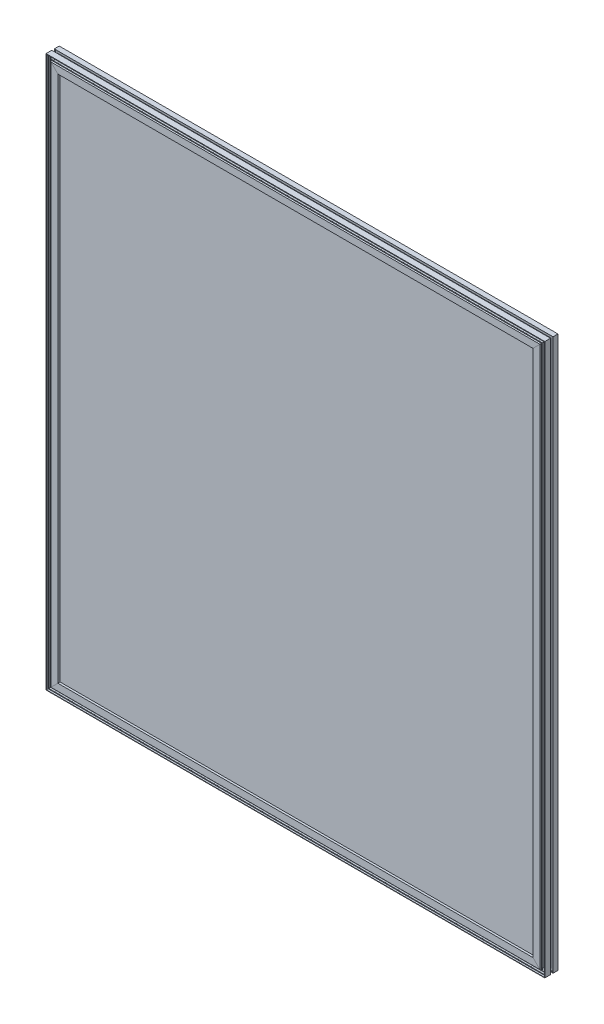
from build123d import *

# Parameters (mm, degrees)
MEMBER_250403_1_DEPTH      = 41.360872141
MEMBER_250403_1_DEPTH_BACK = 1301.360872141
MEMBER_250403_1_2_DEPTH    = 1222.721744282
MEMBER_250403_1_3_DEPTH    = 1342.721744282
MEMBER_250403_1_4_DEPTH    = 1222.721744282
SKETCH_12_W                = 1100
SKETCH_12_H                = 1220
EXTRUDE_1_DEPTH            = 17


with BuildPart() as part:
    # 草图11 → Member 250403_1 (new, two sides: drawn at the far end of the back side and taken through both)
    with BuildSketch(Plane(origin=(-570, 630, 0), x_dir=(1, 0, 0), z_dir=(0, 1, 0)).offset(-MEMBER_250403_1_DEPTH_BACK)):
        with BuildLine():
            Line((11.006838108, 0), (27, 0))
            Line((27, 0), (27, 5))
            Line((27, 5), (25.5, 5))
            Line((25.5, 5), (25.5, 2.2))
            ThreePointArc((25.5, 2.2), (25.207106781, 1.492893219), (24.5, 1.2))
            Line((24.5, 1.2), (18, 1.2))
            ThreePointArc((18, 1.2), (17.292893219, 1.492893219), (17, 2.2))
            Line((17, 2.2), (17, 30))
            Line((17, 30), (12.5, 30))
            Line((12.5, 30), (12.5, 28.8))
            Line((12.5, 28.8), (15.8, 28.8))
            Line((15.8, 28.8), (15.8, 22))
            Line((15.8, 22), (1.2, 22))
            Line((1.2, 22), (1.2, 28.8))
            Line((1.2, 28.8), (4.5, 28.8))
            Line((4.5, 28.8), (4.5, 30))
            Line((4.5, 30), (0, 30))
            Line((0, 30), (0, 18.8))
            Line((0, 18.8), (1.2, 18.8))
            Line((1.2, 18.8), (1.2, 20.8))
            Line((1.2, 20.8), (6.7, 20.8))
            Line((6.7, 20.8), (6.7, 18.8))
            Line((6.7, 18.8), (7.7, 18.8))
            Line((7.7, 18.8), (7.7, 13))
            Line((7.7, 13), (6.7, 13))
            Line((6.7, 13), (6.7, 11))
            Line((6.7, 11), (1.2, 11))
            Line((1.2, 11), (1.2, 13))
            Line((1.2, 13), (0, 13))
            Line((0, 13), (0, 0))
            Line((0, 0), (1.006838108, 0))
            Line((1.006838108, 0), (2.380431303, 2.400675266))
            ThreePointArc((2.380431303, 2.400675266), (2.379848147, 2.600337065), (2.206838108, 2.7))
            Line((2.206838108, 2.7), (1.706838108, 2.7))
            Line((1.706838108, 2.7), (1.706838108, 2.9))
            Line((1.706838108, 2.9), (2.675186721, 3.252126768))
            ThreePointArc((2.675186721, 3.252126768), (2.770651604, 3.325346014), (2.806838108, 3.440085453))
            Line((2.806838108, 3.440085453), (2.806838108, 3.9))
            ThreePointArc((2.806838108, 3.9), (2.748259465, 4.041421356), (2.606838108, 4.1))
            Line((2.606838108, 4.1), (1.006838108, 4.1))
            Line((1.006838108, 4.1), (1.006838108, 9.5))
            ThreePointArc((1.006838108, 9.5), (1.153284718, 9.853553391), (1.506838108, 10))
            Line((1.506838108, 10), (10.506838108, 10))
            ThreePointArc((10.506838108, 10), (10.860391499, 9.853553391), (11.006838108, 9.5))
            Line((11.006838108, 9.5), (11.006838108, 4.1))
            Line((11.006838108, 4.1), (9.406838108, 4.1))
            ThreePointArc((9.406838108, 4.1), (9.265416752, 4.041421356), (9.206838108, 3.9))
            Line((9.206838108, 3.9), (9.206838108, 3.440085453))
            ThreePointArc((9.206838108, 3.440085453), (9.243024613, 3.325346014), (9.338489496, 3.252126768))
            Line((9.338489496, 3.252126768), (10.306838108, 2.9))
            Line((10.306838108, 2.9), (10.306838108, 2.7))
            Line((10.306838108, 2.7), (9.806838108, 2.7))
            ThreePointArc((9.806838108, 2.7), (9.63382807, 2.600337065), (9.633244913, 2.400675266))
            Line((9.633244913, 2.400675266), (11.006838108, 0))
        make_face()
        with BuildLine():
            Line((7.9, 11), (7.9, 11.8))
            ThreePointArc((7.9, 11.8), (8.607106781, 12.092893219), (8.9, 12.8))
            Line((8.9, 12.8), (8.9, 19))
            ThreePointArc((8.9, 19), (8.607106781, 19.707106781), (7.9, 20))
            Line((7.9, 20), (7.9, 20.8))
            Line((7.9, 20.8), (16, 20.8))
            Line((16, 20.8), (16, 1.2))
            Line((16, 1.2), (12.006838108, 1.2))
            Line((12.006838108, 1.2), (12.006838108, 11))
            Line((12.006838108, 11), (7.9, 11))
        make_face(mode=Mode.SUBTRACT)
    extrude(amount=MEMBER_250403_1_DEPTH + MEMBER_250403_1_DEPTH_BACK)

    # Member 250403_1 mitre 1
    split(bisect_by=Plane(origin=(-570, 630, 0), x_dir=(0.707106781, -0.707106781, 0), z_dir=(-0.707106781, -0.707106781, 0)), keep=Keep.TOP)

    # Member 250403_1 mitre 2
    split(bisect_by=Plane(origin=(-570, -630, 0), x_dir=(-0.707106781, -0.707106781, 0), z_dir=(-0.707106781, 0.707106781, 0)), keep=Keep.TOP)


with BuildPart() as body_2:
    # 草图11 on segment 2 (carried to segment 2) → Member 250403_1 2 (new body)
    with BuildSketch(Plane(origin=(611.360872141, -630, 0), x_dir=(0, 1, 0), z_dir=(-1, 0, 0))):
        with BuildLine():
            Line((11.006838108, 0), (27, 0))
            Line((27, 0), (27, 5))
            Line((27, 5), (25.5, 5))
            Line((25.5, 5), (25.5, 2.2))
            ThreePointArc((25.5, 2.2), (25.207106781, 1.492893219), (24.5, 1.2))
            Line((24.5, 1.2), (18, 1.2))
            ThreePointArc((18, 1.2), (17.292893219, 1.492893219), (17, 2.2))
            Line((17, 2.2), (17, 30))
            Line((17, 30), (12.5, 30))
            Line((12.5, 30), (12.5, 28.8))
            Line((12.5, 28.8), (15.8, 28.8))
            Line((15.8, 28.8), (15.8, 22))
            Line((15.8, 22), (1.2, 22))
            Line((1.2, 22), (1.2, 28.8))
            Line((1.2, 28.8), (4.5, 28.8))
            Line((4.5, 28.8), (4.5, 30))
            Line((4.5, 30), (0, 30))
            Line((0, 30), (0, 18.8))
            Line((0, 18.8), (1.2, 18.8))
            Line((1.2, 18.8), (1.2, 20.8))
            Line((1.2, 20.8), (6.7, 20.8))
            Line((6.7, 20.8), (6.7, 18.8))
            Line((6.7, 18.8), (7.7, 18.8))
            Line((7.7, 18.8), (7.7, 13))
            Line((7.7, 13), (6.7, 13))
            Line((6.7, 13), (6.7, 11))
            Line((6.7, 11), (1.2, 11))
            Line((1.2, 11), (1.2, 13))
            Line((1.2, 13), (0, 13))
            Line((0, 13), (0, 0))
            Line((0, 0), (1.006838108, 0))
            Line((1.006838108, 0), (2.380431303, 2.400675266))
            ThreePointArc((2.380431303, 2.400675266), (2.379848147, 2.600337065), (2.206838108, 2.7))
            Line((2.206838108, 2.7), (1.706838108, 2.7))
            Line((1.706838108, 2.7), (1.706838108, 2.9))
            Line((1.706838108, 2.9), (2.675186721, 3.252126768))
            ThreePointArc((2.675186721, 3.252126768), (2.770651604, 3.325346014), (2.806838108, 3.440085453))
            Line((2.806838108, 3.440085453), (2.806838108, 3.9))
            ThreePointArc((2.806838108, 3.9), (2.748259465, 4.041421356), (2.606838108, 4.1))
            Line((2.606838108, 4.1), (1.006838108, 4.1))
            Line((1.006838108, 4.1), (1.006838108, 9.5))
            ThreePointArc((1.006838108, 9.5), (1.153284718, 9.853553391), (1.506838108, 10))
            Line((1.506838108, 10), (10.506838108, 10))
            ThreePointArc((10.506838108, 10), (10.860391499, 9.853553391), (11.006838108, 9.5))
            Line((11.006838108, 9.5), (11.006838108, 4.1))
            Line((11.006838108, 4.1), (9.406838108, 4.1))
            ThreePointArc((9.406838108, 4.1), (9.265416752, 4.041421356), (9.206838108, 3.9))
            Line((9.206838108, 3.9), (9.206838108, 3.440085453))
            ThreePointArc((9.206838108, 3.440085453), (9.243024613, 3.325346014), (9.338489496, 3.252126768))
            Line((9.338489496, 3.252126768), (10.306838108, 2.9))
            Line((10.306838108, 2.9), (10.306838108, 2.7))
            Line((10.306838108, 2.7), (9.806838108, 2.7))
            ThreePointArc((9.806838108, 2.7), (9.63382807, 2.600337065), (9.633244913, 2.400675266))
            Line((9.633244913, 2.400675266), (11.006838108, 0))
        make_face()
        with BuildLine():
            Line((7.9, 11), (7.9, 11.8))
            ThreePointArc((7.9, 11.8), (8.607106781, 12.092893219), (8.9, 12.8))
            Line((8.9, 12.8), (8.9, 19))
            ThreePointArc((8.9, 19), (8.607106781, 19.707106781), (7.9, 20))
            Line((7.9, 20), (7.9, 20.8))
            Line((7.9, 20.8), (16, 20.8))
            Line((16, 20.8), (16, 1.2))
            Line((16, 1.2), (12.006838108, 1.2))
            Line((12.006838108, 1.2), (12.006838108, 11))
            Line((12.006838108, 11), (7.9, 11))
        make_face(mode=Mode.SUBTRACT)
    extrude(amount=MEMBER_250403_1_2_DEPTH)

    # Member 250403_1 2 mitre 1
    split(bisect_by=Plane(origin=(-570, -630, 0), x_dir=(0.707106781, 0.707106781, 0), z_dir=(0.707106781, -0.707106781, 0)), keep=Keep.TOP)

    # Member 250403_1 2 mitre 2
    split(bisect_by=Plane(origin=(570, -630, 0), x_dir=(0.707106781, -0.707106781, 0), z_dir=(-0.707106781, -0.707106781, 0)), keep=Keep.TOP)


with BuildPart() as body_3:
    # 草图11 on segment 3 (carried to segment 3) → Member 250403_1 3 (new body)
    with BuildSketch(Plane(origin=(570, 671.360872141, 0), x_dir=(-1, 0, 0), z_dir=(0, -1, 0))):
        with BuildLine():
            Line((11.006838108, 0), (27, 0))
            Line((27, 0), (27, 5))
            Line((27, 5), (25.5, 5))
            Line((25.5, 5), (25.5, 2.2))
            ThreePointArc((25.5, 2.2), (25.207106781, 1.492893219), (24.5, 1.2))
            Line((24.5, 1.2), (18, 1.2))
            ThreePointArc((18, 1.2), (17.292893219, 1.492893219), (17, 2.2))
            Line((17, 2.2), (17, 30))
            Line((17, 30), (12.5, 30))
            Line((12.5, 30), (12.5, 28.8))
            Line((12.5, 28.8), (15.8, 28.8))
            Line((15.8, 28.8), (15.8, 22))
            Line((15.8, 22), (1.2, 22))
            Line((1.2, 22), (1.2, 28.8))
            Line((1.2, 28.8), (4.5, 28.8))
            Line((4.5, 28.8), (4.5, 30))
            Line((4.5, 30), (0, 30))
            Line((0, 30), (0, 18.8))
            Line((0, 18.8), (1.2, 18.8))
            Line((1.2, 18.8), (1.2, 20.8))
            Line((1.2, 20.8), (6.7, 20.8))
            Line((6.7, 20.8), (6.7, 18.8))
            Line((6.7, 18.8), (7.7, 18.8))
            Line((7.7, 18.8), (7.7, 13))
            Line((7.7, 13), (6.7, 13))
            Line((6.7, 13), (6.7, 11))
            Line((6.7, 11), (1.2, 11))
            Line((1.2, 11), (1.2, 13))
            Line((1.2, 13), (0, 13))
            Line((0, 13), (0, 0))
            Line((0, 0), (1.006838108, 0))
            Line((1.006838108, 0), (2.380431303, 2.400675266))
            ThreePointArc((2.380431303, 2.400675266), (2.379848147, 2.600337065), (2.206838108, 2.7))
            Line((2.206838108, 2.7), (1.706838108, 2.7))
            Line((1.706838108, 2.7), (1.706838108, 2.9))
            Line((1.706838108, 2.9), (2.675186721, 3.252126768))
            ThreePointArc((2.675186721, 3.252126768), (2.770651604, 3.325346014), (2.806838108, 3.440085453))
            Line((2.806838108, 3.440085453), (2.806838108, 3.9))
            ThreePointArc((2.806838108, 3.9), (2.748259465, 4.041421356), (2.606838108, 4.1))
            Line((2.606838108, 4.1), (1.006838108, 4.1))
            Line((1.006838108, 4.1), (1.006838108, 9.5))
            ThreePointArc((1.006838108, 9.5), (1.153284718, 9.853553391), (1.506838108, 10))
            Line((1.506838108, 10), (10.506838108, 10))
            ThreePointArc((10.506838108, 10), (10.860391499, 9.853553391), (11.006838108, 9.5))
            Line((11.006838108, 9.5), (11.006838108, 4.1))
            Line((11.006838108, 4.1), (9.406838108, 4.1))
            ThreePointArc((9.406838108, 4.1), (9.265416752, 4.041421356), (9.206838108, 3.9))
            Line((9.206838108, 3.9), (9.206838108, 3.440085453))
            ThreePointArc((9.206838108, 3.440085453), (9.243024613, 3.325346014), (9.338489496, 3.252126768))
            Line((9.338489496, 3.252126768), (10.306838108, 2.9))
            Line((10.306838108, 2.9), (10.306838108, 2.7))
            Line((10.306838108, 2.7), (9.806838108, 2.7))
            ThreePointArc((9.806838108, 2.7), (9.63382807, 2.600337065), (9.633244913, 2.400675266))
            Line((9.633244913, 2.400675266), (11.006838108, 0))
        make_face()
        with BuildLine():
            Line((7.9, 11), (7.9, 11.8))
            ThreePointArc((7.9, 11.8), (8.607106781, 12.092893219), (8.9, 12.8))
            Line((8.9, 12.8), (8.9, 19))
            ThreePointArc((8.9, 19), (8.607106781, 19.707106781), (7.9, 20))
            Line((7.9, 20), (7.9, 20.8))
            Line((7.9, 20.8), (16, 20.8))
            Line((16, 20.8), (16, 1.2))
            Line((16, 1.2), (12.006838108, 1.2))
            Line((12.006838108, 1.2), (12.006838108, 11))
            Line((12.006838108, 11), (7.9, 11))
        make_face(mode=Mode.SUBTRACT)
    extrude(amount=MEMBER_250403_1_3_DEPTH)

    # Member 250403_1 3 mitre 1
    split(bisect_by=Plane(origin=(570, 630, 0), x_dir=(0.707106781, 0.707106781, 0), z_dir=(0.707106781, -0.707106781, 0)), keep=Keep.TOP)

    # Member 250403_1 3 mitre 2
    split(bisect_by=Plane(origin=(570, -630, 0), x_dir=(-0.707106781, 0.707106781, 0), z_dir=(0.707106781, 0.707106781, 0)), keep=Keep.TOP)


with BuildPart() as body_4:
    # 草图11 on segment 4 (carried to segment 4) → Member 250403_1 4 (new body)
    with BuildSketch(Plane(origin=(-611.360872141, 630, 0), x_dir=(0, -1, 0), z_dir=(1, 0, 0))):
        with BuildLine():
            Line((11.006838108, 0), (27, 0))
            Line((27, 0), (27, 5))
            Line((27, 5), (25.5, 5))
            Line((25.5, 5), (25.5, 2.2))
            ThreePointArc((25.5, 2.2), (25.207106781, 1.492893219), (24.5, 1.2))
            Line((24.5, 1.2), (18, 1.2))
            ThreePointArc((18, 1.2), (17.292893219, 1.492893219), (17, 2.2))
            Line((17, 2.2), (17, 30))
            Line((17, 30), (12.5, 30))
            Line((12.5, 30), (12.5, 28.8))
            Line((12.5, 28.8), (15.8, 28.8))
            Line((15.8, 28.8), (15.8, 22))
            Line((15.8, 22), (1.2, 22))
            Line((1.2, 22), (1.2, 28.8))
            Line((1.2, 28.8), (4.5, 28.8))
            Line((4.5, 28.8), (4.5, 30))
            Line((4.5, 30), (0, 30))
            Line((0, 30), (0, 18.8))
            Line((0, 18.8), (1.2, 18.8))
            Line((1.2, 18.8), (1.2, 20.8))
            Line((1.2, 20.8), (6.7, 20.8))
            Line((6.7, 20.8), (6.7, 18.8))
            Line((6.7, 18.8), (7.7, 18.8))
            Line((7.7, 18.8), (7.7, 13))
            Line((7.7, 13), (6.7, 13))
            Line((6.7, 13), (6.7, 11))
            Line((6.7, 11), (1.2, 11))
            Line((1.2, 11), (1.2, 13))
            Line((1.2, 13), (0, 13))
            Line((0, 13), (0, 0))
            Line((0, 0), (1.006838108, 0))
            Line((1.006838108, 0), (2.380431303, 2.400675266))
            ThreePointArc((2.380431303, 2.400675266), (2.379848147, 2.600337065), (2.206838108, 2.7))
            Line((2.206838108, 2.7), (1.706838108, 2.7))
            Line((1.706838108, 2.7), (1.706838108, 2.9))
            Line((1.706838108, 2.9), (2.675186721, 3.252126768))
            ThreePointArc((2.675186721, 3.252126768), (2.770651604, 3.325346014), (2.806838108, 3.440085453))
            Line((2.806838108, 3.440085453), (2.806838108, 3.9))
            ThreePointArc((2.806838108, 3.9), (2.748259465, 4.041421356), (2.606838108, 4.1))
            Line((2.606838108, 4.1), (1.006838108, 4.1))
            Line((1.006838108, 4.1), (1.006838108, 9.5))
            ThreePointArc((1.006838108, 9.5), (1.153284718, 9.853553391), (1.506838108, 10))
            Line((1.506838108, 10), (10.506838108, 10))
            ThreePointArc((10.506838108, 10), (10.860391499, 9.853553391), (11.006838108, 9.5))
            Line((11.006838108, 9.5), (11.006838108, 4.1))
            Line((11.006838108, 4.1), (9.406838108, 4.1))
            ThreePointArc((9.406838108, 4.1), (9.265416752, 4.041421356), (9.206838108, 3.9))
            Line((9.206838108, 3.9), (9.206838108, 3.440085453))
            ThreePointArc((9.206838108, 3.440085453), (9.243024613, 3.325346014), (9.338489496, 3.252126768))
            Line((9.338489496, 3.252126768), (10.306838108, 2.9))
            Line((10.306838108, 2.9), (10.306838108, 2.7))
            Line((10.306838108, 2.7), (9.806838108, 2.7))
            ThreePointArc((9.806838108, 2.7), (9.63382807, 2.600337065), (9.633244913, 2.400675266))
            Line((9.633244913, 2.400675266), (11.006838108, 0))
        make_face()
        with BuildLine():
            Line((7.9, 11), (7.9, 11.8))
            ThreePointArc((7.9, 11.8), (8.607106781, 12.092893219), (8.9, 12.8))
            Line((8.9, 12.8), (8.9, 19))
            ThreePointArc((8.9, 19), (8.607106781, 19.707106781), (7.9, 20))
            Line((7.9, 20), (7.9, 20.8))
            Line((7.9, 20.8), (16, 20.8))
            Line((16, 20.8), (16, 1.2))
            Line((16, 1.2), (12.006838108, 1.2))
            Line((12.006838108, 1.2), (12.006838108, 11))
            Line((12.006838108, 11), (7.9, 11))
        make_face(mode=Mode.SUBTRACT)
    extrude(amount=MEMBER_250403_1_4_DEPTH)

    # Member 250403_1 4 mitre 1
    split(bisect_by=Plane(origin=(-570, 630, 0), x_dir=(-0.707106781, 0.707106781, 0), z_dir=(0.707106781, 0.707106781, 0)), keep=Keep.TOP)

    # Member 250403_1 4 mitre 2
    split(bisect_by=Plane(origin=(570, 630, 0), x_dir=(-0.707106781, -0.707106781, 0), z_dir=(-0.707106781, 0.707106781, 0)), keep=Keep.TOP)


with BuildPart() as body_5:
    # 草图12 → 凸台-拉伸1 (new body)
    with BuildSketch(Plane(origin=(0, 0, -5), x_dir=(-1, 0, 0), z_dir=(0, 0, -1))):
        Rectangle(SKETCH_12_W, SKETCH_12_H)
    extrude(amount=EXTRUDE_1_DEPTH)


solid = Compound([part.part, body_2.part, body_3.part, body_4.part, body_5.part])
